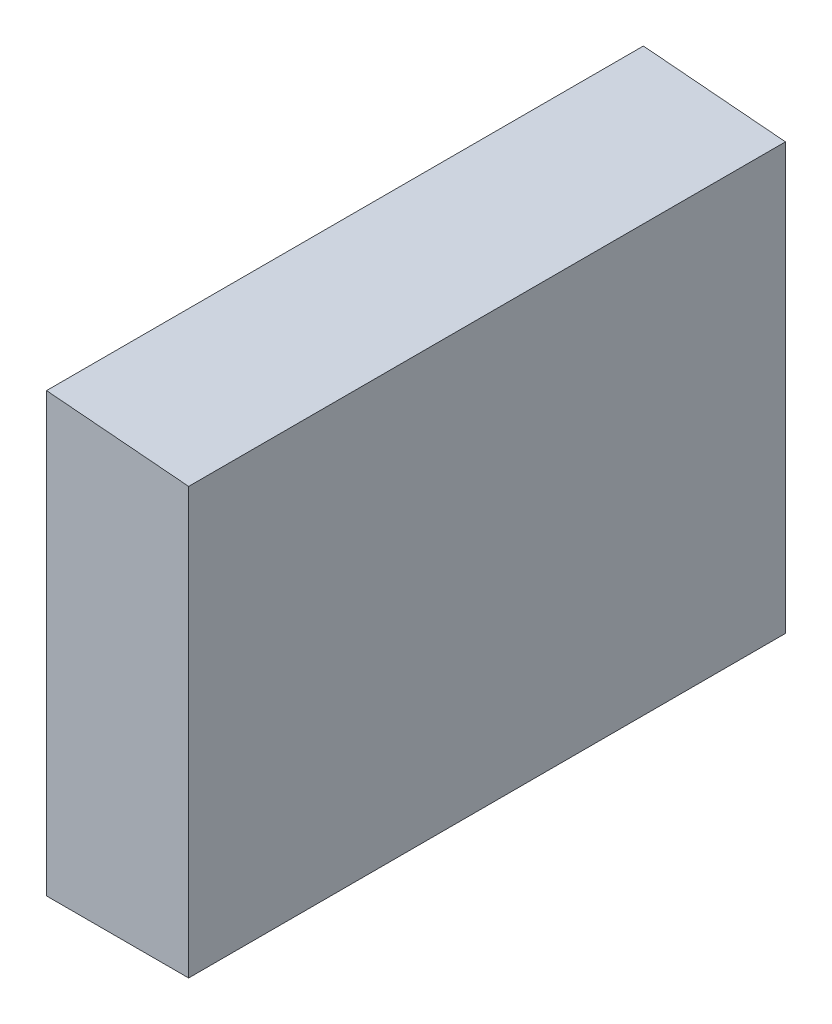
SolidWorks part; units mm, degrees
ref_plane "Front Plane" through (0, 0, 0) normal (0, 0, 1) x (1, 0, 0)
ref_plane "Top Plane" through (0, 0, 0) normal (0, 1, 0) x (1, 0, 0)
ref_plane "Right Plane" through (0, 0, 0) normal (1, 0, 0) x (0, 0, -1)
sketch "Sketch1" plane through (0, 0, 0) normal (0, 0, 1) x (1, 0, 0)
  line L0 (0, 30.8) -> (10, 29.9603)
  line L1 (0, 0) -> (10, 0)
  line L2 (0, 0) -> (0, 30.8)
  line L4 (10, 0) -> (10, 29.9603)
  dimension "D1" = 10
  dimension "D2" = 30.8
  dimension "D3" = 85.2
extrude "Boss-Extrude1" add sketch "Sketch1" along normal blind 42
